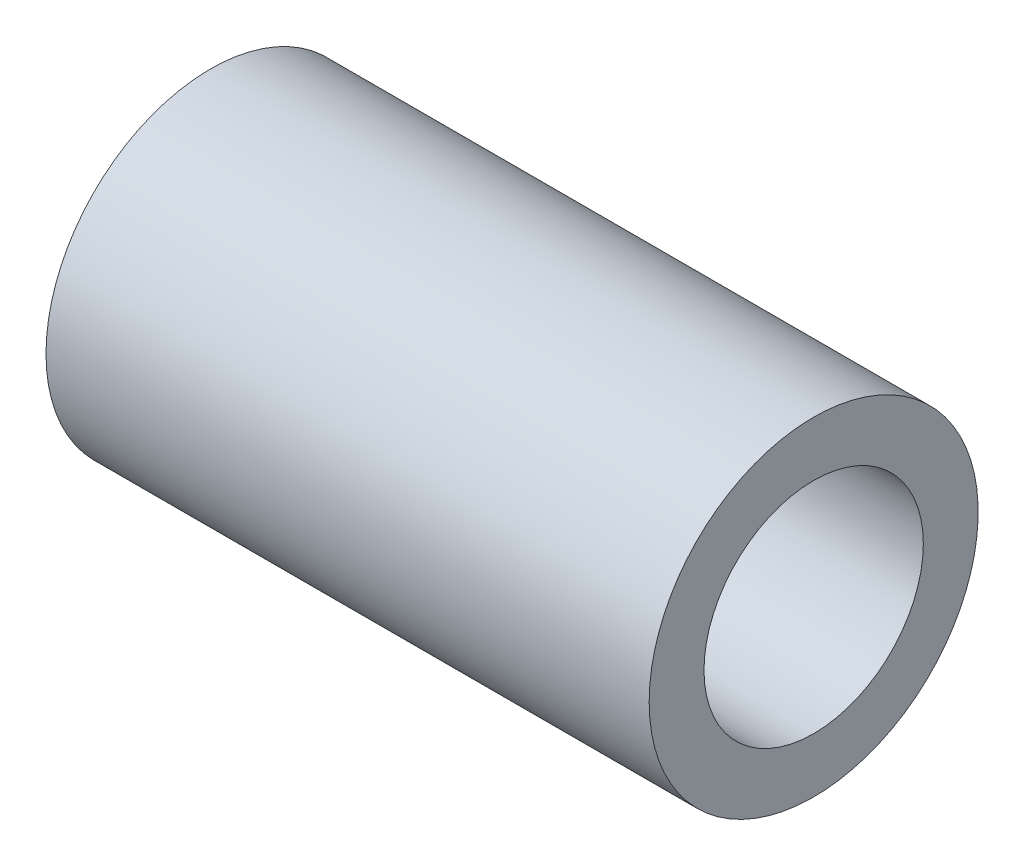
SolidWorks part; units mm, degrees
material "普通碳钢"
ref_plane "前视基准面" through (0, 0, 0) normal (0, 0, 1) x (1, 0, 0)
ref_plane "上视基准面" through (0, 0, 0) normal (0, 1, 0) x (1, 0, 0)
ref_plane "右视基准面" through (0, 0, 0) normal (1, 0, 0) x (0, 0, -1)
other "Configuration Table"
sketch "草图1" plane through (0, 0, 0) normal (0, 0, 1) x (1, 0, 0)
  line L0 (-539.0359, 0) -> (26412.7605, 0) construction
  line L1 (0, 4) -> (0, 6)
  line L2 (0, 6) -> (22, 6)
  line L3 (22, 6) -> (22, 4)
  line L4 (22, 4) -> (0, 4)
  dimension "D1" = 22
  dimension "D2" = 6
  dimension "D3" = 8
revolve "旋转1" add sketch "草图1" angle 360 about L0
